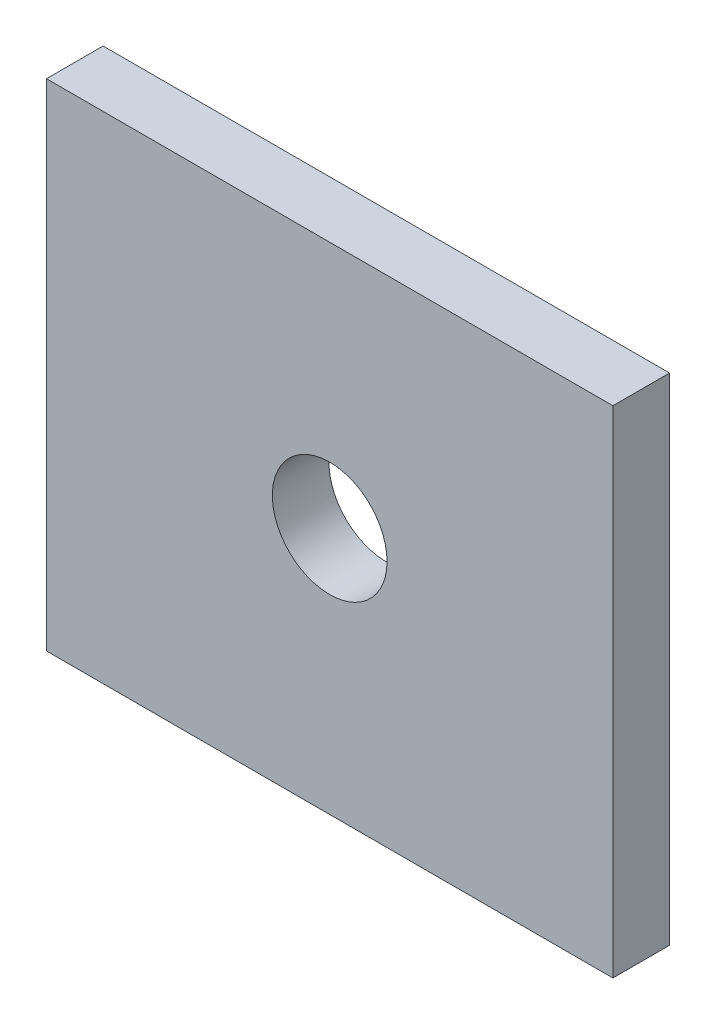
from build123d import *

# Parameters (mm, degrees)
SKETCH_1_W          = 80
SKETCH_1_H          = 70
EXTRUDE_1_DEPTH     = 4
SKETCH_2_R          = 8.1
CUT_EXTRUDE_1_DEPTH = 14


with BuildPart() as part:
    # 草图1 → 凸台-拉伸1 (new, symmetric)
    with BuildSketch(Plane.XY):
        Rectangle(SKETCH_1_W, SKETCH_1_H)
    extrude(amount=EXTRUDE_1_DEPTH, both=True)

    # 草图2 → 切除-拉伸1 (cut, symmetric)
    with BuildSketch(Plane.XY):
        Circle(SKETCH_2_R)
    extrude(amount=CUT_EXTRUDE_1_DEPTH, both=True, mode=Mode.SUBTRACT)


solid = part.part
